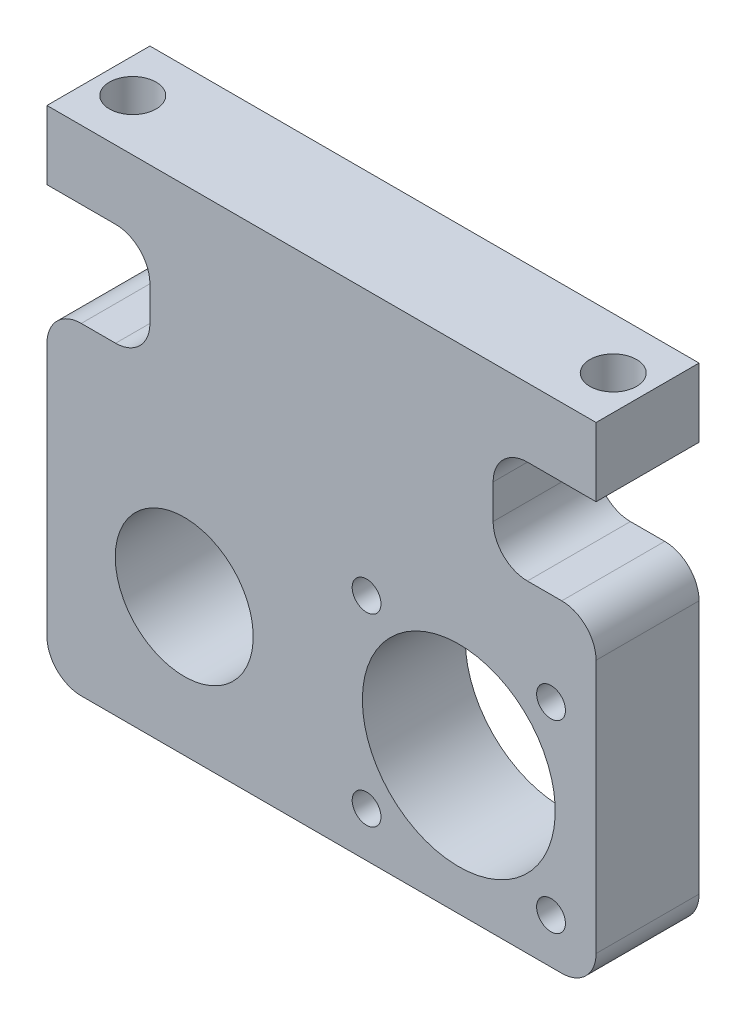
SolidWorks part; units mm, degrees
material "6061合金"
ref_plane "Front Plane" through (0, 0, 0) normal (0, 0, 1) x (1, 0, 0)
ref_plane "Top Plane" through (0, 0, 0) normal (0, 1, 0) x (1, 0, 0)
ref_plane "Right Plane" through (0, 0, 0) normal (1, 0, 0) x (0, 0, -1)
sketch "Sketch1" plane through (0, 0, 0) normal (0, 0, 1) x (1, 0, 0)
  line L0 (0, 0) -> (0, 94.4773) construction
  line L1 (40, 0) -> (-40, 0)
  line L2 (-40, 0) -> (-40, 10)
  line L3 (-40, 10) -> (-25, 10)
  line L7 (40, 10) -> (25, 10)
  line L8 (40, 0) -> (40, 10)
  line L9 (-25, 10) -> (-25, 25)
  line L10 (-25, 25) -> (-40, 25)
  line L11 (-40, 25) -> (-40, 72)
  line L12 (-40, 72) -> (40, 72)
  line L13 (40, 25) -> (40, 72)
  line L14 (25, 25) -> (40, 25)
  line L15 (25, 10) -> (25, 25)
  point P9 (0, 72)
  point P15 (0, 72)
  dimension "D1" = 80
  dimension "D2" = 15
  dimension "D3" = 10
  dimension "D4" = 80
  dimension "D5" = 15
  dimension "D6" = 72
extrude "Boss-Extrude1" add sketch "Sketch1" along normal mid plane 15
sketch "Sketch2" plane through (0, 0, 0) normal (0, -1, 0) x (1, 0, 0)
  line L0 (-40, 0) -> (0, 0) construction
  line L1 (-40, 7.5) -> (-40, -7.5) construction
  line L2 (0, 0) -> (0, 7.5) construction
  line L3 (-40, 7.5) -> (40, 7.5) construction
  circle A0 centre (-35, 0) radius 3.4
  circle A1 centre (35, 0) radius 3.4
  dimension "D1" = 6.8
  dimension "D2" = 5
extrude "Cut-Extrude1" cut sketch "Sketch2" against normal up to next
sketch "Sketch3" plane through (0, 0, 7.5) normal (0, 0, 1) x (1, 0, 0)
  line L0 (-40, 0) -> (40, 0) construction
  line L1 (-20, 52) -> (20, 52) construction
  line L2 (-40, 72) -> (-40, 25) construction
  circle A0 centre (-20, 52) radius 14.05
  circle A1 centre (20, 52) radius 10.05
  dimension "D1" = 20.1
  dimension "D2" = 28.1
  dimension "D3" = 52
  dimension "D5" = 20
  dimension "D4" = 40
extrude "Cut-Extrude2" cut sketch "Sketch3" against normal blind 15
sketch "Sketch4" plane through (0, 0, 7.5) normal (0, 0, 1) x (1, 0, 0)
  line L0 (-1, 52) -> (-20, 52) construction
  line L1 (-20, 52) -> (-6.565, 65.435) construction
  circle A0 centre (-20, 52) radius 19 construction
  circle A1 centre (-6.565, 65.435) radius 1.5
  circle A2 centre (-6.565, 38.565) radius 1.5
  circle A3 centre (-33.435, 38.565) radius 1.5
  circle A4 centre (-33.435, 65.435) radius 1.5
  point P14 (-20, 52)
  dimension "D1" = 38
  dimension "D3" = 3
  dimension "D2" = 45
  dimension "D4" = 4
fillet "Fillet1" radius 5 8 edges at (-25, 10, 0) (-40, 25, 0) (-40, 72, 0) (40, 72, 0) (40, 25, 0) (25, 25, 0) (25, 10, 0) (-25, 25, 0)
hole_wizard "M5 Tapped Hole1" positions "Sketch5" profile "Sketch6" tap size "M5" standard "GB" end condition through all
sketch "Sketch5" plane through (0, 0, -7.5) normal (0, 0, -1) x (-1, 0, 0)
  point P0 (33.435, 38.565)
  point P3 (6.565, 38.565)
  point P6 (6.565, 65.435)
  point P9 (33.435, 65.435)
sketch "Sketch6" plane through (-33.435, 38.565, -7.5) normal (1, 0, 0) x (0, 1, 0)
  line L0 (0, 0) -> (0, 15)
  line L1 (0, 15) -> (2.1, 15)
  line L2 (2.1, 15) -> (2.1, 0)
  line L5 (2.1, 0) -> (0, 0)
  line L11 (0, -6.35) -> (0, 107.95) construction
  dimension "通孔螺纹孔钻头直径" = 4.2
  dimension "通孔螺纹孔钻头深度" = 15
cosmetic thread "Hole Thread1" parameters "D2"=5
cosmetic thread "Hole Thread2" parameters "D2"=5
cosmetic thread "Hole Thread3" parameters "D2"=5
cosmetic thread "Hole Thread4" parameters "D2"=5
move or copy body "Body-Move/Copy1" bodies to move or copy 110 copy no rotation origin (0, 30, 0) rotation axis (0, 0, 1) rotation angle 180
